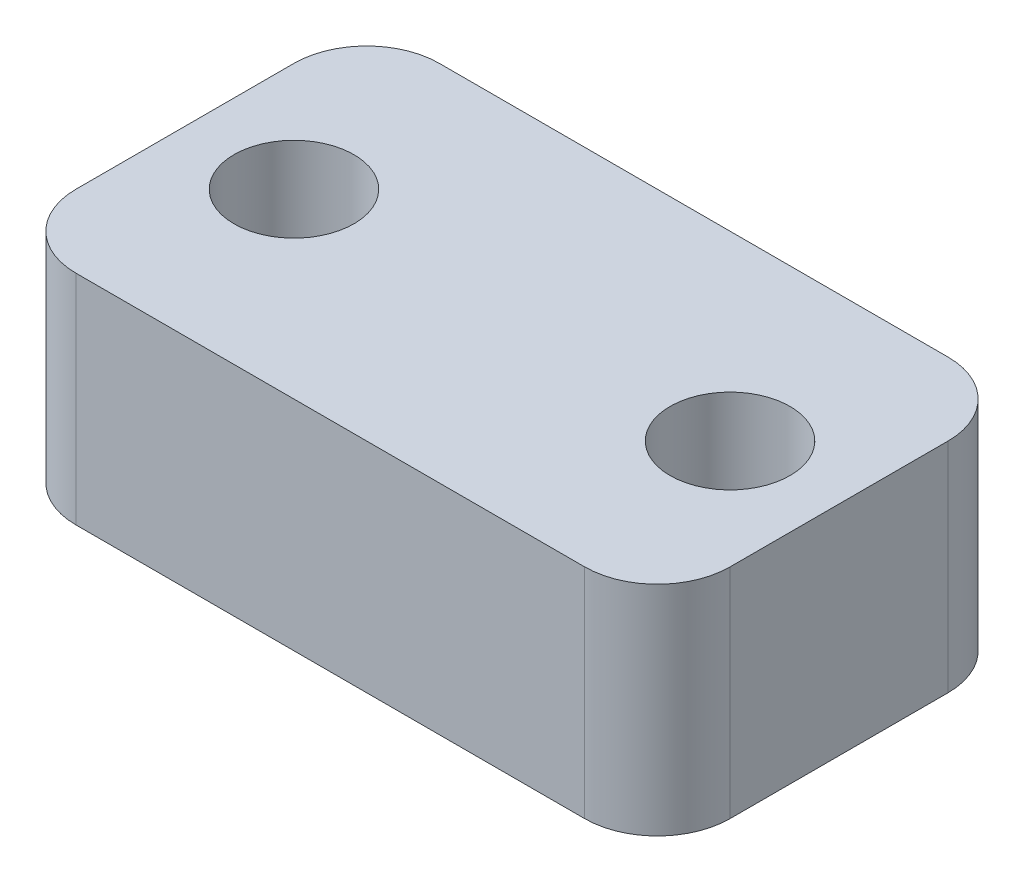
from build123d import *

# Parameters (mm, degrees)
SKETCH_1_W         = 18
SKETCH_1_H         = 6
EXTRUDE_1_DEPTH    = 10
HOLE_WIZARD_M4_3_D = 3.3
FILLET_1_R         = 2


with BuildPart() as part:
    # 草图1 → 凸台-拉伸1 (new body)
    with BuildSketch(Plane.XY):
        Rectangle(SKETCH_1_W, SKETCH_1_H)
    extrude(amount=EXTRUDE_1_DEPTH)

    # M4 螺纹孔3 (through all)
    with Locations(Plane(origin=(0, 3, 0), x_dir=(1, 0, 0), z_dir=(0, 1, 0))):
        with Locations((6, -5), (-6, -5)):
            Hole(HOLE_WIZARD_M4_3_D / 2)

    # 圆角1
    fillet_1_edges = [part.edges().sort_by_distance(p)[0] for p in [
        (-9, 0, 10),
        (9, 0, 10),
        (-9, 0, 0),
        (9, 0, 0),
    ]]
    fillet(fillet_1_edges, radius=FILLET_1_R)


solid = part.part
